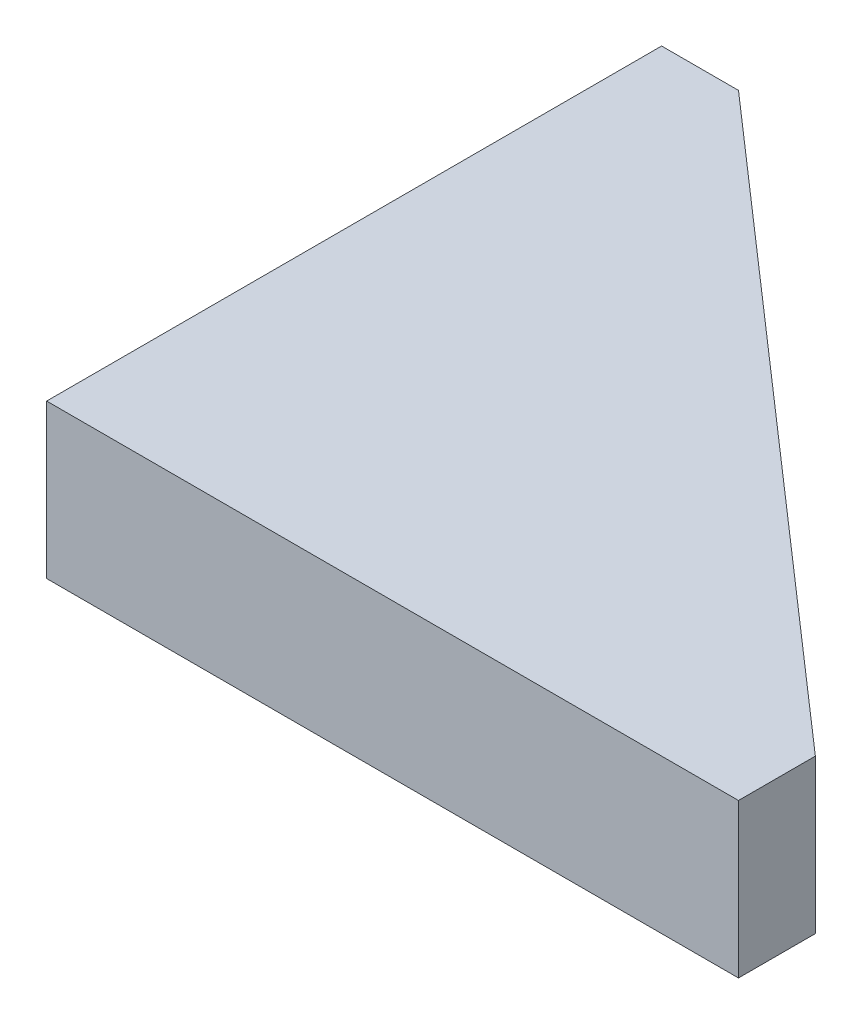
from build123d import *

# Parameters (mm, degrees)
SKETCH_1_W          = 45
SKETCH_1_H          = 40
EXTRUDE_1_DEPTH     = 10
CUT_EXTRUDE_1_DEPTH = 20


with BuildPart() as part:
    # 草图1 → 凸台-拉伸1 (new body)
    with BuildSketch(Plane(origin=(0, 0, 0), x_dir=(1, 0, 0), z_dir=(0, 1, 0))):
        Rectangle(SKETCH_1_W, SKETCH_1_H)
    extrude(amount=EXTRUDE_1_DEPTH)

    # 草图2 → 切除-拉伸1 (cut)
    with BuildSketch(Plane(origin=(0, 10, 0), x_dir=(1, 0, 0), z_dir=(0, 1, 0))):
        Polygon((22.5, 20), (-17.5, 20), (22.5, -15), align=None)
    extrude(amount=-CUT_EXTRUDE_1_DEPTH, mode=Mode.SUBTRACT)


solid = part.part
